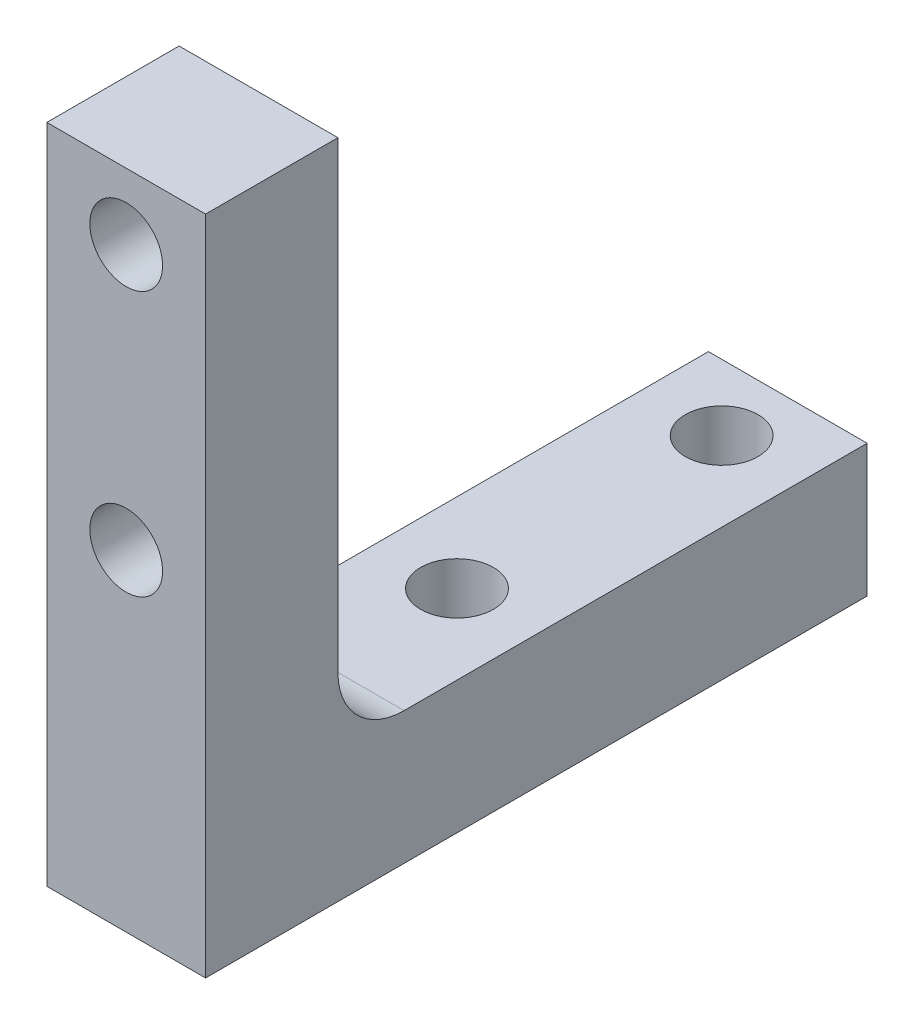
SolidWorks part; units mm, degrees
material "AL6061"
ref_plane "Front Plane" through (0, 0, 0) normal (0, 0, 1) x (1, 0, 0)
ref_plane "Top Plane" through (0, 0, 0) normal (0, 1, 0) x (1, 0, 0)
ref_plane "Right Plane" through (0, 0, 0) normal (1, 0, 0) x (0, 0, -1)
sketch "Sketch1" plane through (0, 0, 0) normal (1, 0, 0) x (0, 0, -1)
  line L0 (0, 0) -> (0, 50)
  line L1 (0, 50) -> (10, 50)
  line L3 (50, 10) -> (50, 0)
  line L4 (50, 0) -> (0, 0)
  line L5 (10, 50) -> (10, 10)
  line L6 (10, 10) -> (50, 10)
  dimension "D1" = 50
  dimension "D2" = 50
  dimension "D3" = 10
  dimension "D4" = 10
extrude "Boss-Extrude1" add sketch "Sketch1" along normal blind 12
fillet "Fillet1" radius 5 1 edges at (6, 10, -10)
hole_wizard "M5 Clearance Hole1" positions "Sketch2" profile "Sketch3" hole size "M5" standard "GB" end condition through all
sketch "Sketch2" plane through (0, 0, -10) normal (0, 0, -1) x (-1, 0, 0)
  line L0 (-6, 50) -> (-6, 0) construction
  line L1 (-12, 50) -> (0, 50) construction
  line L2 (-12, 0) -> (0, 0) construction
  point P9 (-6, 45)
  point P11 (-6, 25)
  dimension "D1" = 25
  dimension "D2" = 20
sketch "Sketch3" plane through (6, 25, -10) normal (1, 0, 0) x (0, 1, 0)
  line L0 (0, 0) -> (0, 10)
  line L1 (0, 10) -> (2.75, 10)
  line L2 (2.75, 10) -> (2.75, 0)
  line L5 (2.75, 0) -> (0, 0)
  line L11 (0, -6.35) -> (0, 107.95) construction
  dimension "通孔孔直径" = 5.5
  dimension "通孔孔深度" = 10
hole_wizard "M5 Clearance Hole2" positions "Sketch4" profile "Sketch5" hole size "M5" standard "GB" end condition through all
sketch "Sketch4" plane through (0, 10, 0) normal (0, 1, 0) x (1, 0, 0)
  line L0 (6, 50) -> (6, 0) construction
  line L1 (12, 50) -> (0, 50) construction
  line L2 (12, 0) -> (0, 0) construction
  point P9 (6, 25)
  point P11 (6, 45)
  dimension "D1" = 25
  dimension "D2" = 20
sketch "Sketch5" plane through (6, 10, -45) normal (1, 0, 0) x (0, 0, 1)
  line L0 (0, 0) -> (0, 10)
  line L1 (0, 10) -> (2.75, 10)
  line L2 (2.75, 10) -> (2.75, 0)
  line L5 (2.75, 0) -> (0, 0)
  line L11 (0, -6.35) -> (0, 107.95) construction
  dimension "通孔孔直径" = 5.5
  dimension "通孔孔深度" = 10
